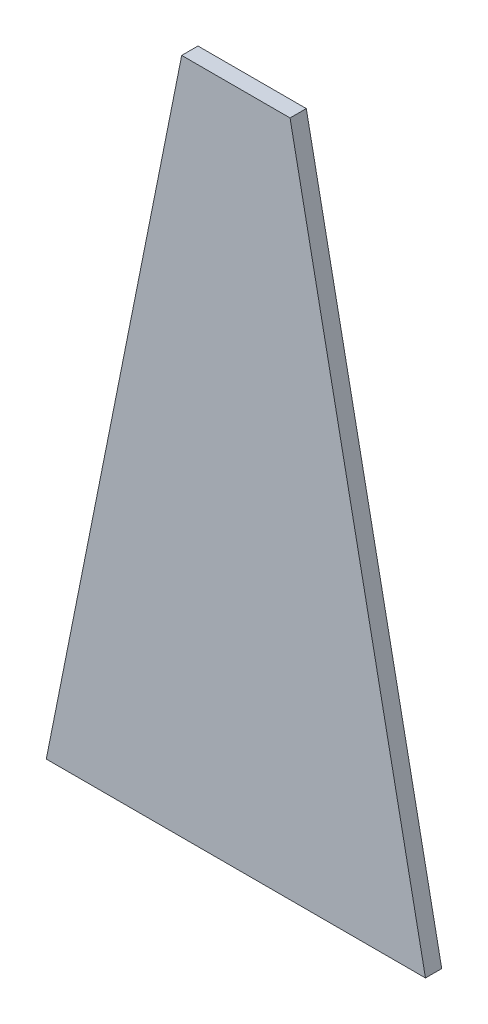
from build123d import *

# Parameters (mm, degrees)
SKETCH_1_W          = 280
SKETCH_1_H          = 500
EXTRUDE_1_DEPTH     = 12
SKETCH_2_OUTSIDE_W  = 396.638
SKETCH_2_OUTSIDE_H  = 616.638
CUT_EXTRUDE_1_DEPTH = 12


with BuildPart() as part:
    # 草图1 → 凸台-拉伸1 (new body)
    with BuildSketch(Plane.XY):
        Rectangle(SKETCH_1_W, SKETCH_1_H)
    extrude(amount=EXTRUDE_1_DEPTH)

    # 草图2 outside → 切除-拉伸1 (cut)
    with BuildSketch(Plane.XY.offset(12)):
        Rectangle(SKETCH_2_OUTSIDE_W, SKETCH_2_OUTSIDE_H)
        Polygon((-140, -250), (-40, 250), (40, 250), (140, -250), align=None, mode=Mode.SUBTRACT)
    extrude(amount=-CUT_EXTRUDE_1_DEPTH, mode=Mode.SUBTRACT)


solid = part.part
